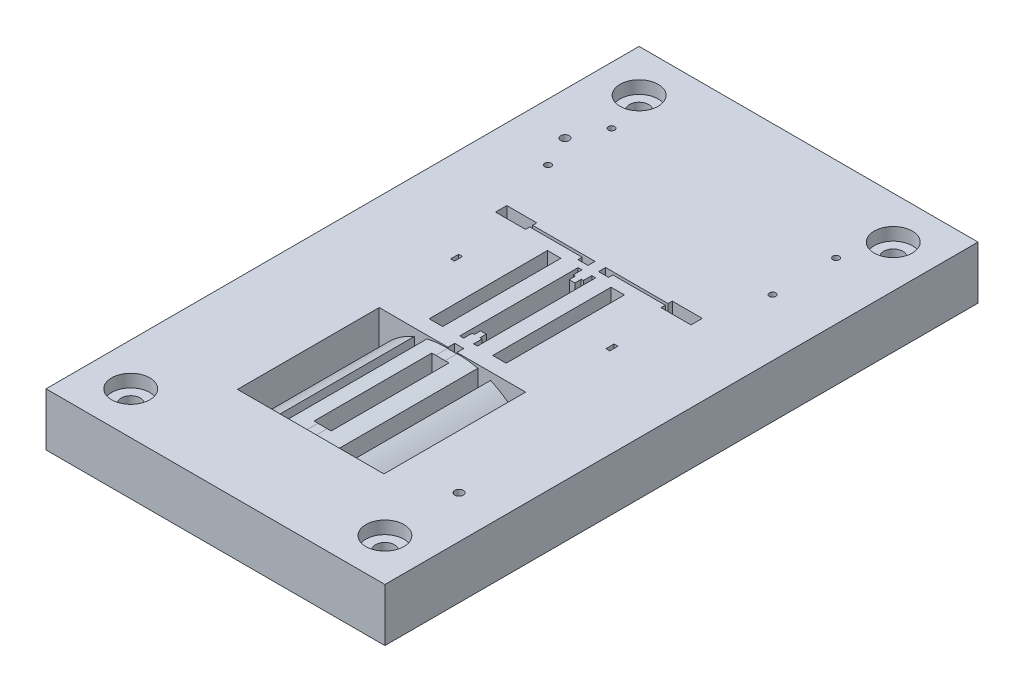
SolidWorks part; units mm, degrees
ref_plane "Front Plane" through (0, 0, 0) normal (0, 0, 1) x (1, 0, 0)
ref_plane "Top Plane" through (0, 0, 0) normal (0, 1, 0) x (1, 0, 0)
ref_plane "Right Plane" through (0, 0, 0) normal (1, 0, 0) x (0, 0, -1)
sketch "Sketch1" plane through (0, 0, 0) normal (0, 1, 0) x (1, 0, 0)
  line L0 (0, 0) -> (0, 58.6327) construction
  line L1 (-80, 0) -> (80, 0)
  line L2 (80, 0) -> (80, -280)
  line L3 (80, -280) -> (-80, -280)
  line L4 (-80, 0) -> (-80, -280)
  dimension "D1" = 280
extrude "Boss-Extrude1" add sketch "Sketch1" against normal blind 25
ref_plane "Plane1" through (0, 0, 235) normal (0, 0, 1) x (1, 0, 0)
hole_wizard "CBORE for M8 Pan Head Machine Screw1" positions "Sketch6" profile "Sketch5" counterbore size "M8" standard "ANSI Metric" end condition through all
sketch "Sketch6" plane through (0, 0, 0) normal (0, 1, 0) x (1, 0, 0)
  line L0 (-80, 0) -> (-80, -280)
  line L1 (-80, -280) -> (80, -280)
  line L2 (80, -280) -> (80, 0)
  line L3 (80, 0) -> (-80, 0)
  point P38 (60, -260)
  point P39 (60, -20)
  point P40 (-60, -20)
  point P41 (-60, -260)
sketch "Sketch5" plane through (-60, 0, 260) normal (1, 0, 0) x (0, 0, 1)
  line L0 (0, 0) -> (0, 25)
  line L1 (0, 25) -> (4.5, 25)
  line L3 (4.5, 25) -> (4.5, 6)
  line L4 (4.5, 6) -> (9, 6)
  line L5 (9, 6) -> (9, 0)
  line L7 (9, 0) -> (0, 0)
  line L11 (0, -6.35) -> (0, 107.95) construction
  dimension "Thru Hole Dia." = 9
  dimension "Thru Hole Depth" = 25
  dimension "C'Bore Dia." = 18
  dimension "C'Bore Depth" = 6
ref_plane "Plane2" through (0, 0, 0) normal (1, 0, 0) x (0, 0, -1)
ref_plane "基准面1" through (0, 0, 240.93) normal (0, 0, 1) x (1, 0, 0)
sketch "Sketch4" plane through (0, 0, 240.93) normal (0, 0, 1) x (1, 0, 0)
  line L0 (-29.5253, -19.27) -> (-29.5253, -11.1549)
  line L1 (-34.5722, -17.6206) -> (-30.6203, -19.9022)
  line L2 (-34.5722, 0) -> (-34.5722, -17.6206)
  line L4 (34.5722, -17.6206) -> (34.5722, 0)
  line L5 (30.6203, -19.9022) -> (34.5722, -17.6206)
  line L6 (29.5253, -11.1549) -> (29.5253, -19.27)
  line L7 (-2.2069, -0.5) -> (2.2069, -0.5)
  line L25 (-80, 0) -> (80, 0) construction
  line L26 (-34.5722, 0) -> (34.5722, 0)
  arc A0 (-2.2069, -0.5) -> (-29.5253, -11.1549) centre (-3.08, -38.61) ccw
  arc A1 (-30.6203, -19.9022) -> (-29.5253, -19.27) centre (-30.2553, -19.27) ccw
  arc A2 (29.5253, -19.27) -> (30.6203, -19.9022) centre (30.2553, -19.27) ccw
  arc A3 (29.5253, -11.1549) -> (2.2069, -0.5) centre (3.08, -38.61) ccw
extrude "Cut-Extrude2" cut sketch "Sketch4" against normal blind 72.8 contours A3 L6 A2 L5 L4 L26 L2 L1 A1 L0 A0 L7
sketch "草图5" plane through (0, 0, 0) normal (0, 1, 0) x (1, 0, 0)
  line L45 (2.12, -164.91) -> (-2.12, -164.91)
  line L47 (-2.12, -164.91) -> (-2.12, -168.25)
  line L53 (2.12, -168.25) -> (-2.12, -168.25)
  line L55 (2.12, -164.91) -> (2.12, -168.25)
  line L57 (4.06, -229.42) -> (4.06, -173.8)
  line L59 (4.06, -173.8) -> (-4.06, -173.8)
  line L61 (-4.06, -173.8) -> (-4.06, -229.42)
  line L63 (-4.06, -229.42) -> (4.06, -229.42)
  line L136 (35.77, -127.58) -> (37.61, -127.58)
  line L137 (37.61, -131.42) -> (37.61, -127.58)
  line L138 (35.77, -131.42) -> (37.61, -131.42)
  line L139 (35.77, -131.42) -> (35.77, -127.58)
  line L140 (18.17, -160.92) -> (18.17, -105.08)
  line L141 (11.83, -105.08) -> (18.17, -105.08)
  line L142 (11.83, -160.92) -> (11.83, -105.08)
  line L143 (11.83, -160.92) -> (18.17, -160.92)
  line L144 (4.39, -104.86) -> (4.39, -160.7)
  line L145 (4.39, -160.7) -> (2.55, -160.7)
  line L146 (2.55, -156.7) -> (2.55, -160.7)
  line L147 (1.55, -156.7) -> (2.55, -156.7)
  line L148 (1.55, -153.7) -> (1.55, -156.7)
  line L149 (-1.11, -153.7) -> (1.55, -153.7)
  line L150 (-1.11, -156.7) -> (-1.11, -153.7)
  line L151 (-2.11, -156.7) -> (-1.11, -156.7)
  line L152 (-2.11, -160.7) -> (-2.11, -156.7)
  line L153 (-2.11, -160.7) -> (-3.95, -160.7)
  line L154 (-3.95, -104.86) -> (-3.95, -160.7)
  line L155 (-2.11, -104.86) -> (-3.95, -104.86)
  line L156 (-2.11, -108.86) -> (-2.11, -104.86)
  line L157 (-1.11, -108.86) -> (-2.11, -108.86)
  line L158 (-1.11, -111.86) -> (-1.11, -108.86)
  line L159 (1.55, -111.86) -> (-1.11, -111.86)
  line L160 (1.55, -108.86) -> (1.55, -111.86)
  line L161 (2.55, -108.86) -> (1.55, -108.86)
  line L162 (2.55, -104.86) -> (2.55, -108.86)
  line L163 (4.39, -104.86) -> (2.55, -104.86)
  line L164 (-11.83, -105.08) -> (-11.83, -160.92)
  line L165 (-11.83, -160.92) -> (-18.17, -160.92)
  line L166 (-18.17, -105.08) -> (-18.17, -160.92)
  line L167 (-11.83, -105.08) -> (-18.17, -105.08)
  line L168 (-35.77, -127.58) -> (-35.77, -131.42)
  line L169 (-35.77, -131.42) -> (-37.61, -131.42)
  line L170 (-37.61, -127.58) -> (-37.61, -131.42)
  line L171 (-35.77, -127.58) -> (-37.61, -127.58)
  line L172 (7.25, -101.64) -> (2.5, -101.64)
  line L173 (2.5, -98.3) -> (2.5, -101.64)
  line L174 (31.99, -98.3) -> (2.5, -98.3)
  line L175 (31.99, -96.3) -> (31.99, -98.3)
  line L176 (46.14, -96.3) -> (31.99, -96.3)
  line L177 (46.14, -101.64) -> (46.14, -96.3)
  line L178 (46.14, -101.64) -> (31.99, -101.64)
  line L179 (31.99, -99.64) -> (31.99, -101.64)
  line L180 (7.25, -99.64) -> (31.99, -99.64)
  line L181 (7.25, -101.64) -> (7.25, -99.64)
  line L182 (-2.5, -98.3) -> (-31.99, -98.3)
  line L183 (-31.99, -98.3) -> (-31.99, -96.3)
  line L184 (-31.99, -96.3) -> (-46.14, -96.3)
  line L185 (-46.14, -96.3) -> (-46.14, -101.64)
  line L186 (-31.99, -101.64) -> (-46.14, -101.64)
  line L187 (-31.99, -101.64) -> (-31.99, -99.64)
  line L188 (-31.99, -99.64) -> (-7.25, -99.64)
  line L189 (-7.25, -99.64) -> (-7.25, -101.64)
  line L190 (-2.5, -101.64) -> (-7.25, -101.64)
  line L191 (-2.5, -98.3) -> (-2.5, -101.64)
extrude "Cut-Extrude4" cut sketch "草图5" against normal up to next
sketch "草图6" plane through (0, 0, 0) normal (0, 1, 0) x (1, 0, 0)
  line L0 (-18, -168.13) -> (-18, -240.93)
  line L1 (-34.5722, -168.13) -> (-2.12, -168.13) construction
  line L2 (-34.5722, -240.93) -> (34.5722, -240.93) construction
  line L3 (-18, -240.93) -> (-12, -240.93)
  line L4 (-12, -240.93) -> (-12, -168.13)
  line L5 (-12, -168.13) -> (-18, -168.13)
  line L6 (0, -164.91) -> (0, -263.8592) construction
  line L7 (2.12, -164.91) -> (-2.12, -164.91) construction
  line L8 (-15, -168.13) -> (-15, -244.0821) construction
  line L9 (12, -240.93) -> (12, -168.13)
  line L10 (18, -240.93) -> (12, -240.93)
  line L11 (18, -168.13) -> (18, -240.93)
  line L12 (12, -168.13) -> (18, -168.13)
  dimension "D1" = 12
  dimension "D2" = 6
extrude "Cut-Extrude5" cut sketch "草图6" against normal blind 15
sketch "Sketch7" plane through (0, 0, 240.93) normal (0, 0, -1) x (-1, 0, 0)
  line L0 (-33.9068, 0) -> (34.5722, 0)
  line L14 (-18, -3.5311) -> (-18, -15)
  line L15 (-18, -15) -> (-12, -15)
  line L16 (-12, -15) -> (-12, -1.5483)
  line L17 (-2.2069, -0.5) -> (2.2069, -0.5)
  line L18 (12, -1.5483) -> (12, -15)
  line L19 (12, -15) -> (18, -15)
  line L20 (18, -15) -> (18, -3.5311)
  line L21 (29.5253, -11.1549) -> (29.5253, -19.27)
  line L22 (30.6203, -19.9022) -> (34.5722, -17.6206)
  line L23 (34.5722, -17.6206) -> (34.5722, 0)
  line L24 (34.5722, 0) -> (-34.5722, 0)
  line L25 (-34.5722, 0) -> (-34.5722, -17.6206)
  line L26 (-34.5722, -17.6206) -> (-30.6203, -19.9022)
  line L27 (-29.5253, -19.27) -> (-29.5253, -11.1549)
  line L28 (-18, -3.5311) -> (-18, -15)
  line L29 (-18, -15) -> (-12, -15)
  line L30 (-12, -15) -> (-12, -1.5483)
  line L31 (-2.2069, -0.5) -> (2.2069, -0.5)
  line L32 (12, -1.5483) -> (12, -15)
  line L33 (12, -15) -> (18, -15)
  line L34 (18, -15) -> (18, -3.5311)
  line L35 (29.5253, -11.1549) -> (29.5253, -19.27)
  line L36 (30.6203, -19.9022) -> (34.5722, -17.6206)
  line L37 (34.5722, -17.6206) -> (34.5722, 0)
  line L38 (34.5722, 0) -> (-34.5722, 0)
  line L39 (-34.5722, 0) -> (-34.5722, -17.6206)
  line L40 (-34.5722, -17.6206) -> (-30.6203, -19.9022)
  line L41 (-29.5253, -19.27) -> (-29.5253, -11.1549)
  arc A6 (-18, -3.5311) -> (-29.5253, -11.1549) centre (-3.08, -38.61) ccw
  arc A7 (-2.2069, -0.5) -> (-12, -1.5483) centre (-3.08, -38.61) ccw
  arc A8 (12, -1.5483) -> (2.2069, -0.5) centre (3.08, -38.61) ccw
  arc A9 (29.5253, -11.1549) -> (18, -3.5311) centre (3.08, -38.61) ccw
  arc A10 (29.5253, -19.27) -> (30.6203, -19.9022) centre (30.2553, -19.27) ccw
  arc A11 (-30.6203, -19.9022) -> (-29.5253, -19.27) centre (-30.2553, -19.27) ccw
  arc A12 (-18, -3.5311) -> (-29.5253, -11.1549) centre (-3.08, -38.61) ccw
  arc A13 (-2.2069, -0.5) -> (-12, -1.5483) centre (-3.08, -38.61) ccw
  arc A14 (12, -1.5483) -> (2.2069, -0.5) centre (3.08, -38.61) ccw
  arc A15 (29.5253, -11.1549) -> (18, -3.5311) centre (3.08, -38.61) ccw
  arc A16 (29.5253, -19.27) -> (30.6203, -19.9022) centre (30.2553, -19.27) ccw
  arc A17 (-30.6203, -19.9022) -> (-29.5253, -19.27) centre (-30.2553, -19.27) ccw
  dimension "D1" = 0
extrude "凸台-拉伸1" add sketch "Sketch7" along normal blind 5.9 contours L38 L39 L40 A17 L41 A12 L28 L29 L30 A13 L31 A14 L32 L33 L34 A15 L35 A16 L36 L37
sketch "Sketch10" plane through (0, 0, 0) normal (0, 1, 0) x (1, 0, 0)
  line L0 (-15, -165.7763) -> (-15, -235.03) construction
  line L1 (0, -168.25) -> (0, -200.4075) construction
  line L2 (-2.12, -168.25) -> (2.12, -168.25) construction
  circle A0 centre (-15, -184.86) radius 2.5
  circle A1 centre (-15, -218.315) radius 2.5
  circle A2 centre (-15, -201.585) radius 2.5
  circle A3 centre (15, -218.315) radius 2.5
  circle A4 centre (15, -201.585) radius 2.5
  circle A5 centre (15, -184.86) radius 2.5
  dimension "D2" = 5
  dimension "D3" = 16.725
  dimension "D4" = 16.73
extrude "Cut-Extrude6" cut sketch "Sketch10" against normal blind 20
sketch "Sketch12" plane through (0, 0, 0) normal (0, 0, -1) x (-1, 0, 0)
  line L0 (0, 0) -> (0, 18.5082) construction
sketch "Sketch13" plane through (0, 0, 0) normal (0, 1, 0) x (1, 0, 0)
  line L0 (80, 0) -> (-80, 0) construction
  line L1 (53.003, -69.9966) -> (53.003, -127.4687) construction
  line L2 (-53.003, -69.9966) -> (-53.003, -121.8343) construction
  line L3 (0, 0) -> (0, -83.5884) construction
  line L12 (7.25, -99.64) -> (31.99, -99.64)
  line L13 (7.25, -101.64) -> (7.25, -99.64)
  line L14 (2.5, -101.64) -> (7.25, -101.64)
  line L15 (2.5, -98.3) -> (2.5, -101.64)
  line L16 (31.99, -98.3) -> (2.5, -98.3)
  line L17 (31.99, -96.3) -> (31.99, -98.3)
  line L18 (46.14, -96.3) -> (31.99, -96.3)
  line L19 (46.14, -101.64) -> (46.14, -96.3)
  line L20 (31.99, -101.64) -> (46.14, -101.64)
  line L21 (31.99, -99.64) -> (31.99, -101.64)
  line L22 (7.25, -99.64) -> (31.99, -99.64)
  line L23 (7.25, -101.64) -> (7.25, -99.64)
  line L24 (2.5, -101.64) -> (7.25, -101.64)
  line L25 (2.5, -98.3) -> (2.5, -101.64)
  line L26 (31.99, -98.3) -> (2.5, -98.3)
  line L27 (31.99, -96.3) -> (31.99, -98.3)
  line L28 (46.14, -96.3) -> (31.99, -96.3)
  line L29 (46.14, -101.64) -> (46.14, -96.3)
  line L30 (31.99, -101.64) -> (46.14, -101.64)
  line L31 (31.99, -99.64) -> (31.99, -101.64)
  line L32 (-2.5, -98.3) -> (-31.99, -98.3)
  line L33 (-2.5, -101.64) -> (-2.5, -98.3)
  line L34 (-7.25, -101.64) -> (-2.5, -101.64)
  line L35 (-7.25, -99.64) -> (-7.25, -101.64)
  line L36 (-31.99, -99.64) -> (-7.25, -99.64)
  line L37 (-31.99, -101.64) -> (-31.99, -99.64)
  line L38 (-46.14, -101.64) -> (-31.99, -101.64)
  line L39 (-46.14, -96.3) -> (-46.14, -101.64)
  line L40 (-31.99, -96.3) -> (-46.14, -96.3)
  line L41 (-31.99, -98.3) -> (-31.99, -96.3)
  line L42 (-2.5, -98.3) -> (-31.99, -98.3)
  line L43 (-2.5, -101.64) -> (-2.5, -98.3)
  line L44 (-7.25, -101.64) -> (-2.5, -101.64)
  line L45 (-7.25, -99.64) -> (-7.25, -101.64)
  line L46 (-31.99, -99.64) -> (-7.25, -99.64)
  line L47 (-31.99, -101.64) -> (-31.99, -99.64)
  line L48 (-46.14, -101.64) -> (-31.99, -101.64)
  line L49 (-46.14, -96.3) -> (-46.14, -101.64)
  line L50 (-31.99, -96.3) -> (-46.14, -96.3)
  line L51 (-31.99, -98.3) -> (-31.99, -96.3)
  circle A0 centre (-53.003, -40) radius 1.5
  circle A1 centre (-53.003, -69.9966) radius 1.5
  circle A2 centre (53.003, -69.9966) radius 1.5
  circle A3 centre (53.003, -40) radius 1.5
  dimension "D1" = 53.003
  dimension "D5" = 3
  dimension "D2" = 29.9966
  dimension "D3" = 40
  dimension "D4" = 53.003
  dimension "D6" = 0
  dimension "D7" = 0
extrude "Cut-Extrude7" cut sketch "Sketch13" against normal blind 8
ref_plane "基准面2" through (0, 0, 0) normal (1, 0, 0) x (0, 0, -1)
sketch "Sketch14" plane through (0, -25, 0) normal (0, -1, 0) x (1, 0, 0)
  line L0 (60, 260) -> (60, 20) construction
  line L1 (-60, 260) -> (-60, 20) construction
  circle A0 centre (-60, 55) radius 2
  circle A1 centre (60, 225) radius 2
  dimension "D1" = 4
  dimension "D2" = 35
  dimension "D3" = 35
extrude "Cut-Extrude8" cut sketch "Sketch14" against normal through all
